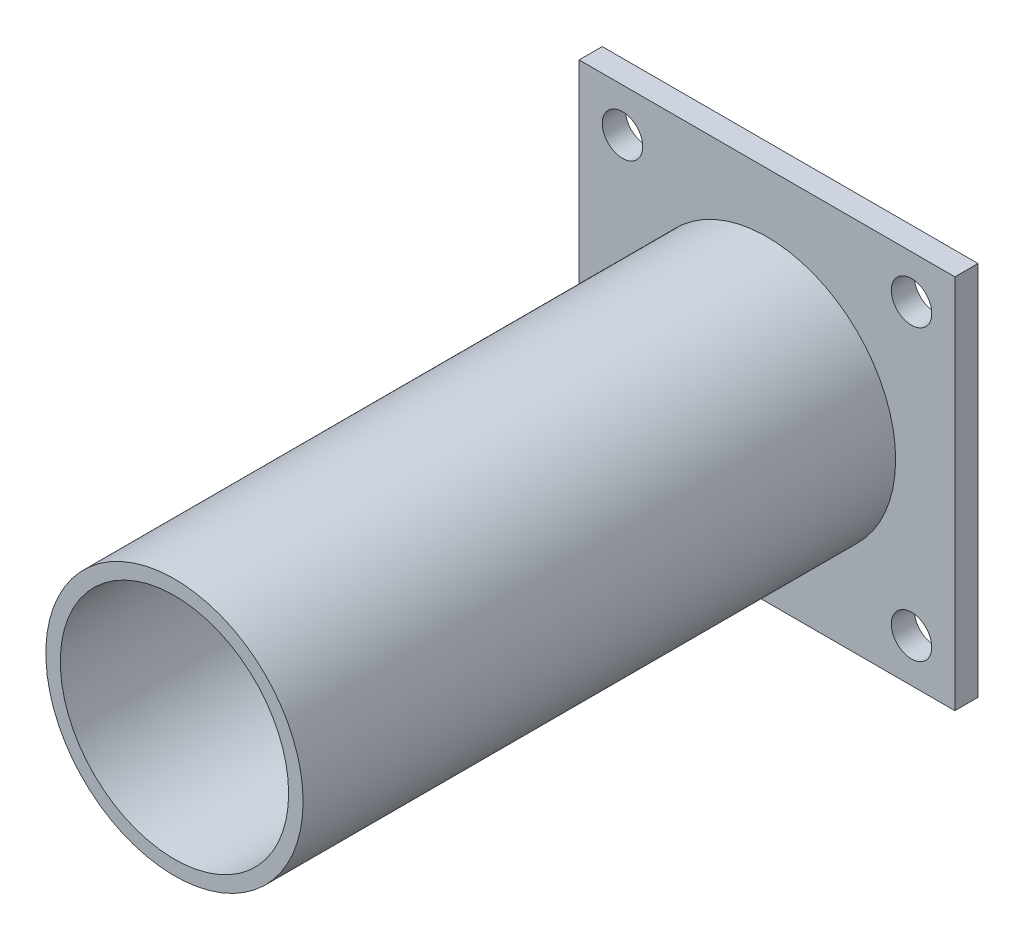
SolidWorks part; units mm, degrees
material "XRAAT"
ref_plane "前视基准面" through (0, 0, 0) normal (0, 0, 1) x (1, 0, 0)
ref_plane "上视基准面" through (0, 0, 0) normal (0, 1, 0) x (1, 0, 0)
ref_plane "右视基准面" through (0, 0, 0) normal (1, 0, 0) x (0, 0, -1)
sketch "草图2" plane through (0, 0, 0) normal (0, 0, 1) x (1, 0, 0)
  line L0 (0, 65) -> (0, 0) construction
  line L1 (65, -65) -> (-65, -65)
  line L2 (65, -65) -> (65, 65)
  line L3 (65, 65) -> (-65, 65)
  line L4 (-65, -65) -> (-65, 65)
  line L5 (65, -65) -> (-65, 65) construction
  line L6 (65, 65) -> (-65, -65) construction
  line L7 (0, 0) -> (-65, 0) construction
  circle A0 centre (-50, 50) radius 7
  circle A1 centre (50, 50) radius 7
  circle A2 centre (50, -50) radius 7
  circle A3 centre (-50, -50) radius 7
  point P0 (0, 0)
  dimension "D2" = 14
  dimension "D3" = 100
  dimension "D1" = 130
extrude "凸台-拉伸1" add sketch "草图2" along normal blind 8
sketch "草图3" plane through (0, 0, 0) normal (0, 1, 0) x (1, 0, 0)
  line L0 (0, -8) -> (0, -213)
  line L1 (65, -8) -> (-65, -8) construction
  dimension "D1" = 205
other "圆管 89X5(1)"
ref_plane "基准面2" through (0, 0, 8) normal (0, 0, 1) x (1, 0, 0)
sketch "Sketch12" plane through (0, 0, 8) normal (0, 0, 1) x (1, 0, 0)
  circle A0 centre (0, 0) radius 39.5
  circle A1 centre (0, 0) radius 44.5
  point P3 (0, 0)
  dimension "Out_dia" = 89
  dimension "D1" = 5
